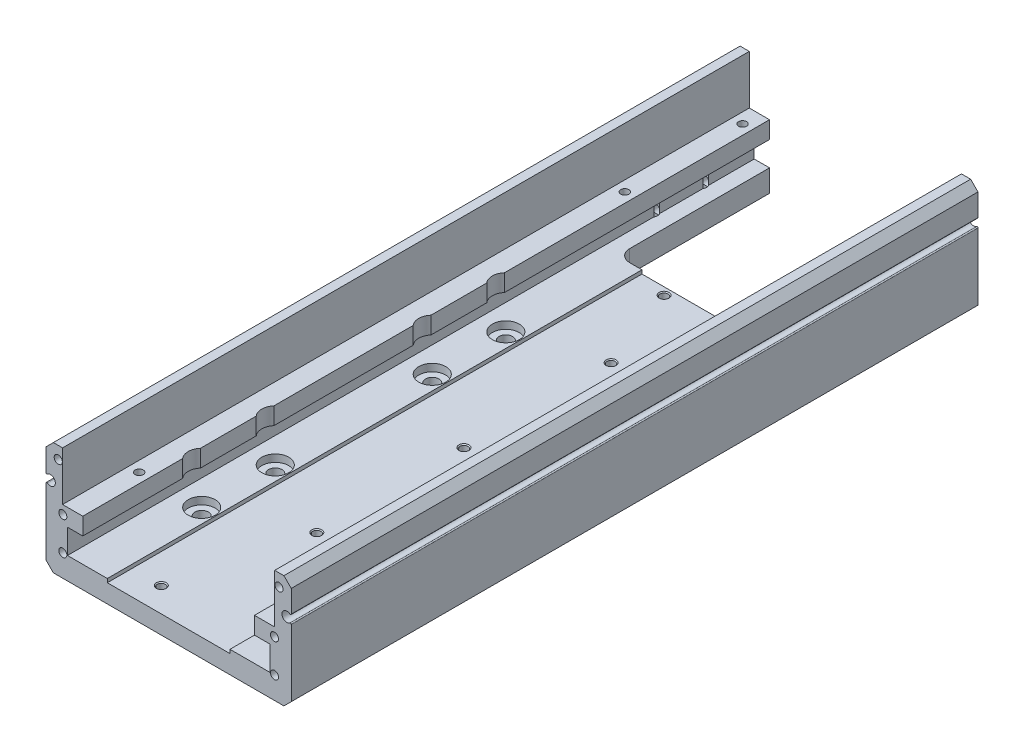
SolidWorks part; units mm, degrees
material "6061 合金"
ref_plane "前视基准面" through (0, 0, 0) normal (0, 0, 1) x (1, 0, 0)
ref_plane "上视基准面" through (0, 0, 0) normal (0, 1, 0) x (1, 0, 0)
ref_plane "右视基准面" through (0, 0, 0) normal (1, 0, 0) x (0, 0, -1)
sketch "草图1" plane through (0, 0, 0) normal (0, 0, 1) x (1, 0, 0)
  line L1 (-50, 23) -> (50, 23)
  line L2 (-50, 23) -> (-50, -23)
  line L3 (-50, -23) -> (50, -23)
  line L4 (50, 23) -> (50, -23)
  line L5 (-50, 23) -> (50, -23) construction
  line L6 (-50, -23) -> (50, 23) construction
  point P0 (0, 0)
  dimension "D1" = 100
  dimension "D2" = 46
extrude "凸台-拉伸1" add sketch "草图1" along normal mid plane 280
chamfer "倒角1" distance 3 angle 45 4 edges at (50, 23, 0) (50, -23, 0) (-50, 23, 0) (-50, -23, 0)
sketch "草图2" plane through (0, 0, 0) normal (0, 0, 1) x (1, 0, 0)
  line L0 (0, 23) -> (0, -23) construction
  line L1 (47, 23) -> (-47, 23) construction
  line L2 (-47, -23) -> (47, -23) construction
  line L3 (43.25, 23) -> (-43.25, 23)
  line L4 (-43.25, 23) -> (-43.25, 3)
  line L5 (-43.25, 3) -> (-35, 3)
  line L6 (-35, 3) -> (-35, -4)
  line L7 (-35, -4) -> (-41.25, -4)
  line L8 (-41.25, -4) -> (-41.25, -14)
  line L9 (-41.25, -14) -> (-25, -14)
  line L10 (-25, -14) -> (-25, -15.5)
  line L11 (-25, -15.5) -> (25, -15.5)
  line L12 (43.25, 23) -> (43.25, 3)
  line L13 (43.25, 3) -> (35, 3)
  line L14 (35, 3) -> (35, -4)
  line L15 (35, -4) -> (41.25, -4)
  line L16 (41.25, -4) -> (41.25, -14)
  line L17 (41.25, -14) -> (25, -14)
  line L18 (25, -14) -> (25, -15.5)
  point P23 (0, -15.5)
  dimension "D1" = 50
  dimension "D2" = 7.5
  dimension "D3" = 9
  dimension "D4" = 82.5
  dimension "D5" = 70
  dimension "D6" = 86.5
  dimension "D7" = 10
  dimension "D8" = 7
extrude "切除-拉伸1" cut sketch "草图2" against normal through all both and the other way through all
sketch "草图3" plane through (0, 0, 0) normal (0, 0, 1) x (1, 0, 0)
  line L0 (0, -25.5404) -> (0, 0) construction
  line L1 (-47, -23) -> (47, -23) construction
  circle A0 centre (-43.15, -14) radius 1.6
  circle A1 centre (-45, 18) radius 1.6
  circle A2 centre (43.15, -14) radius 1.6
  circle A3 centre (45, 18) radius 1.6
  dimension "D2" = 86.3
  dimension "D3" = 3.2
  dimension "D4" = 32
  dimension "D1" = 9
  dimension "D5" = 90
extrude "切除-拉伸2" cut sketch "草图3" against normal through all both and the other way through all
sketch "草图4" plane through (0, 0, 0) normal (0, 0, 1) x (1, 0, 0)
  line L0 (0, 0) -> (0, -23.0913) construction
  line L1 (-43.25, 23) -> (-47, 23) construction
  line L2 (-50, 20) -> (-50, -20) construction
  circle A0 centre (-48.2, 9.1) radius 2
  circle A1 centre (48.2, 9.1) radius 2
  dimension "D2" = 1.8
  dimension "D3" = 4
  dimension "D1" = 13.9
extrude "切除-拉伸3" cut sketch "草图4" against normal through all both and the other way through all
sketch "草图5" plane through (0, -23, 0) normal (0, -1, 0) x (1, 0, 0)
  line L0 (0, -140) -> (0, 140) construction
  line L1 (-47, -140) -> (47, -140) construction
  line L2 (-47, 140) -> (47, 140) construction
  line L4 (-35, -78) -> (35, -78)
  line L5 (-35, -78) -> (-35, -140)
  line L6 (-35, -140) -> (35, -140)
  line L7 (35, -78) -> (35, -140)
  line L8 (-35, -78) -> (35, -140) construction
  line L9 (-35, -140) -> (35, -78) construction
  point P6 (0, -109)
  dimension "D1" = 70
  dimension "D2" = 62
extrude "切除-拉伸4" cut sketch "草图5" against normal through all
hole_wizard "M4 螺纹孔4" positions "草图7" profile "草图6" tap size "M4" standard "GB"
sketch "草图7" plane through (0, 0, 140) normal (0, 0, 1) x (1, 0, 0)
  line L0 (-43.15, -14) -> (-43.15, 0) construction
  line L5 (-35, -0.5) -> (-43.15, -0.5) construction
  line L6 (-35, 3) -> (-35, -4) construction
  point P20 (-43.15, -0.5)
sketch "草图6" plane through (-43.15, -0.5, 140) normal (1, 0, 0) x (0, -1, 0)
  line L0 (0, 0) -> (0, 15.9914)
  line L1 (0, 15.9914) -> (1.65, 15)
  line L2 (1.65, 15) -> (1.65, 0)
  line L5 (1.65, 0) -> (0, 0)
  line L10 (0, 15.9914) -> (-1.65, 15) construction
  line L11 (0, -6.35) -> (0, 107.95) construction
  dimension "螺纹孔钻头直径" = 3.3
  dimension "螺纹孔钻头深度" = 15
  dimension "导头角度" = 118
cosmetic thread "孔螺蚊线1" parameters "D1"=15, "D2"=4
mirror "镜向1" about plane through (0, 0, 0) normal (1, 0, 0) of "M4 螺纹孔4"
mirror "镜向2" about plane through (0, 0, 0) normal (0, 0, 1) of "M4 螺纹孔4", "镜向1"
hole_wizard "M4 螺纹孔1" positions "草图9" profile "草图8" tap size "M4" standard "GB"
sketch "草图9" plane through (0, 0, 140) normal (0, 0, 1) x (1, 0, 0)
  point P0 (-43.15, -14)
  point P3 (-45, 18)
  point P6 (45, 18)
  point P9 (43.15, -14)
sketch "草图8" plane through (-43.15, -14, 140) normal (1, 0, 0) x (0, -1, 0)
  line L0 (0, 0) -> (0, 12.9914)
  line L1 (0, 12.9914) -> (1.65, 12)
  line L2 (1.65, 12) -> (1.65, 0)
  line L5 (1.65, 0) -> (0, 0)
  line L10 (0, 12.9914) -> (-1.65, 12) construction
  line L11 (0, -6.35) -> (0, 107.95) construction
  dimension "螺纹孔钻头直径" = 3.3
  dimension "螺纹孔钻头深度" = 12
  dimension "导头角度" = 118
cosmetic thread "孔螺蚊线2" parameters "D1"=10, "D2"=4
cosmetic thread "孔螺蚊线3" parameters "D1"=10, "D2"=4
cosmetic thread "孔螺蚊线4" parameters "D1"=10, "D2"=4
cosmetic thread "孔螺蚊线5" parameters "D1"=10, "D2"=4
mirror "镜向3" about plane through (0, 0, 0) normal (0, 0, 1) of "M4 螺纹孔1"
fillet "圆角1" radius 5 2 edges at (35, -18.5, -78) (-35, -18.5, -78)
hole_wizard "M4 螺纹孔2" positions "草图11" profile "草图10" tap size "M4" standard "GB"
sketch "草图11" plane through (0, 3, 0) normal (0, 1, 0) x (1, 0, 0)
  line L0 (-39, 133) -> (-39, 85) construction
  line L1 (-39, 85) -> (-39, -113) construction
  line L3 (-43.25, -140) -> (-35, -140) construction
  line L4 (-43.25, 140) -> (-35, 140) construction
  point P0 (-39, 133)
  point P2 (-39, 85)
  point P4 (-39, -113)
  dimension "D1" = 27
  dimension "D2" = 7
  dimension "D3" = 48
  dimension "D4" = 39
sketch "草图10" plane through (-39, 3, -133) normal (1, 0, 0) x (0, 0, 1)
  line L0 (0, 0) -> (0, 26)
  line L1 (0, 26) -> (1.65, 26)
  line L2 (1.65, 26) -> (1.65, 0)
  line L5 (1.65, 0) -> (0, 0)
  line L11 (0, -6.35) -> (0, 20.821) construction
  dimension "通孔螺纹孔钻头直径" = 3.3
  dimension "通孔螺纹孔钻头深度" = 26
cosmetic thread "孔螺蚊线6" parameters "D2"=4
cosmetic thread "孔螺蚊线7" parameters "D2"=4
cosmetic thread "孔螺蚊线8" parameters "D2"=4
mirror "镜向4" about plane through (0, 0, 0) normal (1, 0, 0) of "M4 螺纹孔2"
fillet "圆角2" radius 0.35 4 edges at (-50, 8.2282, 0) (-50, 9.9718, 0) (50, 9.9718, 0) (50, 8.2282, 0)
sketch "草图14" plane through (0, -23, 0) normal (0, -1, 0) x (1, 0, 0)
  line L0 (-47, 140) -> (47, 140) construction
  line L1 (-35, 601.9002) -> (35, 601.9002)
  line L2 (-35, 601.9002) -> (-35, 65)
  line L3 (-35, 65) -> (35, 65)
  line L4 (35, 601.9002) -> (35, 65)
  line L5 (-35, 601.9002) -> (35, 65) construction
  line L6 (-35, 65) -> (35, 601.9002) construction
  point P0 (0, 333.4501)
  dimension "D1" = 70
  dimension "D2" = 75
extrude "切除-拉伸5" [suppressed] cut sketch "草图14" against normal through all
fillet "圆角3" [suppressed] radius 5
hole_wizard "M5 六角头螺栓的柱形沉头孔1" positions "3D草图1" profile "草图16" counterbore size "M5" standard "GB" end condition through all
sketch3d "3D草图1"
  line L2 (0, 0, 0) -> (0, 0, -119.4054) construction
  line L4 (25, -15.5, -78) -> (-25, -15.5, -78) construction
  point P17 (30.8545, 3, -28.3336)
  point P19 (-30.8545, 3, -28.3336)
  dimension "D1" = 31
  dimension "D3" = 53
  dimension "D2" = 31
  dimension "D4" = 53
sketch "草图16" plane through (30.8545, 3, -28.3336) normal (1, 0, 0) x (0, 0, 1)
  line L0 (0, 0) -> (0, 26)
  line L1 (0, 26) -> (2.75, 26)
  line L3 (2.75, 26) -> (2.75, 20)
  line L4 (2.75, 20) -> (5.5, 20)
  line L5 (5.5, 20) -> (5.5, 0)
  line L7 (5.5, 0) -> (0, 0)
  line L11 (0, -6.35) -> (0, 107.95) construction
  dimension "通孔孔直径" = 5.5
  dimension "通孔孔深度" = 26
  dimension "柱形沉头孔直径" = 11
  dimension "柱形沉头孔深度" = 20
pattern_linear "阵列(线性)1" count 2 spacing 94 along (0, 0, 1) of "M5 六角头螺栓的柱形沉头孔1"
pattern_linear "阵列(线性)2" count 2 spacing 30 along (0, 0, 1) of "M5 六角头螺栓的柱形沉头孔1", "阵列(线性)1"
sketch "草图17" plane through (0, -15.5, 0) normal (0, 1, 0) x (1, 0, 0)
  circle A0 centre (0, 40.4) radius 0.7281
  circle A1 centre (0, -79.6) radius 0.8536
  circle A2 centre (0, -19.6) radius 0.861
extrude "切除-拉伸6" cut sketch "草图17" against normal blind 33
sketch "草图18" plane through (0, -15.5, 0) normal (0, 1, 0) x (1, 0, 0)
  line L0 (-25, 78) -> (-25, -140) construction
  line L1 (-25, -140) -> (25, -140) construction
  circle A0 centre (-13, -130) radius 1.0555
  dimension "D2" = 10
  dimension "D1" = 12
extrude "切除-拉伸7" cut sketch "草图18" against normal blind 33
hole_wizard "M4 螺纹孔5" positions "3D草图2" profile "草图19" tap size "M4" standard "GB"
sketch3d "3D草图2"
  line L1 (0, -23, 79.6) -> (0, -15.5, 79.6) construction
  line L2 (0, -23, 19.6) -> (0, -15.5, 19.6) construction
  line L3 (0, -23, -40.4) -> (0, -15.5, -40.4) construction
  point P4 (0, -15.5, 79.6)
  point P8 (0, -15.5, 19.6)
  point P12 (0, -15.5, -40.4)
sketch "草图19" plane through (0, -15.5, 79.6) normal (1, 0, 0) x (0, 0, 1)
  line L0 (0, 0) -> (0, 12.4914)
  line L1 (0, 12.4914) -> (1.65, 11.5)
  line L2 (1.65, 11.5) -> (1.65, 0.375)
  line L3 (1.65, 0.375) -> (2.025, 0)
  line L5 (2.025, 0) -> (0, 0)
  line L6 (-1.65, 0.375) -> (-2.025, 0) construction
  line L10 (0, 12.4914) -> (-1.65, 11.5) construction
  line L11 (0, -6.35) -> (0, 107.95) construction
  dimension "螺纹孔钻头直径" = 3.3
  dimension "螺纹孔钻头深度" = 11.5
  dimension "近端锥形沉头孔直径" = 4.05
  dimension "近端锥形沉头孔角度" = 90
  dimension "导头角度" = 118
hole_wizard "M4 螺纹孔6" positions "3D草图3" profile "草图20" tap size "M4" standard "GB"
sketch3d "3D草图3"
  line L0 (-13, -23, 130) -> (-13, -15.5, 130) construction
  point P0 (-13, -15.5, 130)
sketch "草图20" plane through (-13, -15.5, 130) normal (1, 0, 0) x (0, 0, 1)
  line L0 (0, 0) -> (0, 12.4914)
  line L1 (0, 12.4914) -> (1.65, 11.5)
  line L2 (1.65, 11.5) -> (1.65, 0.375)
  line L3 (1.65, 0.375) -> (2.025, 0)
  line L5 (2.025, 0) -> (0, 0)
  line L6 (-1.65, 0.375) -> (-2.025, 0) construction
  line L10 (0, 12.4914) -> (-1.65, 11.5) construction
  line L11 (0, -6.35) -> (0, 107.95) construction
  dimension "螺纹孔钻头直径" = 3.3
  dimension "螺纹孔钻头深度" = 11.5
  dimension "近端锥形沉头孔直径" = 4.05
  dimension "近端锥形沉头孔角度" = 90
  dimension "导头角度" = 118
pattern_linear "阵列(线性)3" count 2 spacing 205 along (0, 0, -1) of "M4 螺纹孔6"
hole_wizard "M5 螺纹孔1" positions "草图21" profile "草图22" tap size "M5" standard "GB"
sketch "草图21" plane through (0, -23, 0) normal (0, -1, 0) x (-1, 0, 0)
  point P0 (-43, 120.2644)
  point P2 (-43, 100.2644)
sketch "草图22" plane through (43, -23, -120.2644) normal (1, 0, 0) x (0, 0, -1)
  line L0 (0, 0) -> (0, 15.2618)
  line L1 (0, 15.2618) -> (2.1, 14)
  line L2 (2.1, 14) -> (2.1, 0)
  line L5 (2.1, 0) -> (0, 0)
  line L10 (0, 15.2618) -> (-2.1, 14) construction
  line L11 (0, -6.35) -> (0, 107.95) construction
  dimension "螺纹孔钻头直径" = 4.2
  dimension "螺纹孔钻头深度" = 14
  dimension "导头角度" = 118
cosmetic thread "孔螺蚊线9" parameters "D1"=10, "D2"=5
cosmetic thread "孔螺蚊线10" parameters "D1"=10, "D2"=5
mirror "镜向5" about plane through (0, 0, 0) normal (1, 0, 0) of "M5 螺纹孔1"
